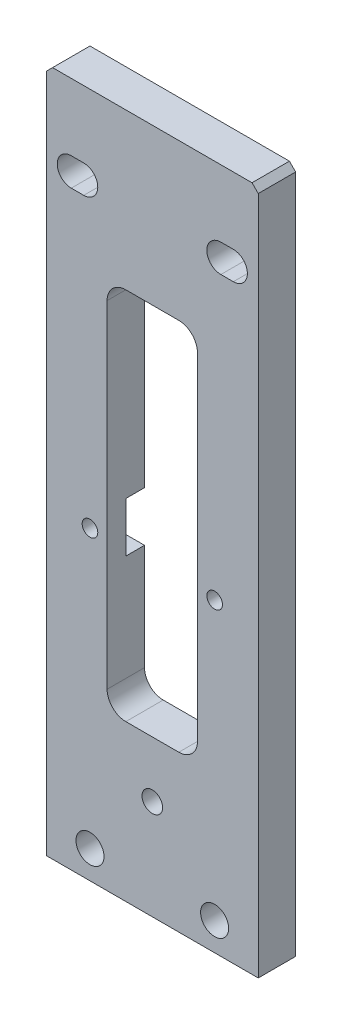
from build123d import *

# Parameters (mm, degrees)
SKETCH1_W                  = 34
SKETCH1_H                  = 110
BOSS_EXTRUDE1_DEPTH        = 6
CHAMFER1_SIZE              = 1
F_4_5_4_5_DIAMETER_HOLE1_D = 4.5
CUT_EXTRUDE1_DEPTH         = 58.879184514
SKETCH12_W                 = 14.5
SKETCH12_H                 = 60
CUT_EXTRUDE2_DEPTH         = 58.879184514
SKETCH13_W                 = 27
SKETCH13_H                 = 8
CUT_EXTRUDE3_DEPTH         = 3
FILLET1_R                  = 3
SKETCH14_R                 = 1
CUT_EXTRUDE4_DEPTH         = 3
M3_TAPPED_HOLE1_D          = 2.5
M4_TAPPED_HOLE1_D          = 3.3


with BuildPart() as part:
    # Sketch1 → Boss-Extrude1 (new body)
    with BuildSketch(Plane.XY):
        Rectangle(SKETCH1_W, SKETCH1_H)
    extrude(amount=BOSS_EXTRUDE1_DEPTH)

    # Chamfer1
    chamfer1_edges = [part.edges().sort_by_distance(p)[0] for p in [
        (-17, 55, 3),
        (17, 55, 3),
    ]]
    chamfer(chamfer1_edges, length=CHAMFER1_SIZE)

    # Ø4.5 (4.5) Diameter Hole1 (through all)
    with Locations(Plane(origin=(0, 0, 0), x_dir=(-1, 0, 0), z_dir=(0, 0, -1))):
        with Locations((-10, -50.5), (10, -50.5)):
            Hole(F_4_5_4_5_DIAMETER_HOLE1_D / 2)

    # Sketch4 → Cut-Extrude1 (cut, through all)
    with BuildSketch(Plane(origin=(0, 0, 0), x_dir=(-1, 0, 0), z_dir=(0, 0, -1))):
        with BuildLine():
            Line((-13, 44.25), (-11, 44.25))
            ThreePointArc((-11, 44.25), (-8.75, 42), (-11, 39.75))
            Line((-11, 39.75), (-13, 39.75))
            ThreePointArc((-13, 39.75), (-15.25, 42), (-13, 44.25))
        make_face()
        with BuildLine():
            Line((11, 44.25), (13, 44.25))
            ThreePointArc((13, 44.25), (15.25, 42), (13, 39.75))
            Line((13, 39.75), (11, 39.75))
            ThreePointArc((11, 39.75), (8.75, 42), (11, 44.25))
        make_face()
    extrude(amount=-CUT_EXTRUDE1_DEPTH, mode=Mode.SUBTRACT)

    # Sketch12 → Cut-Extrude2 (cut, through all)
    with BuildSketch(Plane(origin=(0, 0, 0), x_dir=(-1, 0, 0), z_dir=(0, 0, -1))):
        Rectangle(SKETCH12_W, SKETCH12_H)
    extrude(amount=-CUT_EXTRUDE2_DEPTH, mode=Mode.SUBTRACT)

    # Sketch13 → Cut-Extrude3 (cut)
    with BuildSketch(Plane(origin=(0, 0, 0), x_dir=(-1, 0, 0), z_dir=(0, 0, -1))):
        with Locations((0, -6)):
            Rectangle(SKETCH13_W, SKETCH13_H)
    extrude(amount=-CUT_EXTRUDE3_DEPTH, mode=Mode.SUBTRACT)

    # Fillet1
    fillet1_edges = [part.edges().sort_by_distance(p)[0] for p in [
        (-7.25, 30, 3),
        (-7.25, -30, 3),
        (7.25, -30, 3),
        (7.25, 30, 3),
    ]]
    fillet(fillet1_edges, radius=FILLET1_R)

    # Sketch14 → Cut-Extrude4 (cut)
    with BuildSketch(Plane(origin=(0, 0, 0), x_dir=(-1, 0, 0), z_dir=(0, 0, -1))):
        with Locations((-13.5, -2)):
            Circle(SKETCH14_R)
        with Locations((-13.5, -10)):
            Circle(SKETCH14_R)
        with Locations((13.5, -10)):
            Circle(SKETCH14_R)
        with Locations((13.5, -2)):
            Circle(SKETCH14_R)
    extrude(amount=-CUT_EXTRUDE4_DEPTH, mode=Mode.SUBTRACT)

    # M3 Tapped Hole1 (through all)
    with Locations(Plane(origin=(0, 0, 0), x_dir=(-1, 0, 0), z_dir=(0, 0, -1))):
        with Locations((-10, -6), (10, -6)):
            Hole(M3_TAPPED_HOLE1_D / 2)

    # M4 Tapped Hole1 (through all)
    with Locations(Plane.XY.offset(6)):
        with Locations((0, -39)):
            Hole(M4_TAPPED_HOLE1_D / 2)


solid = part.part
